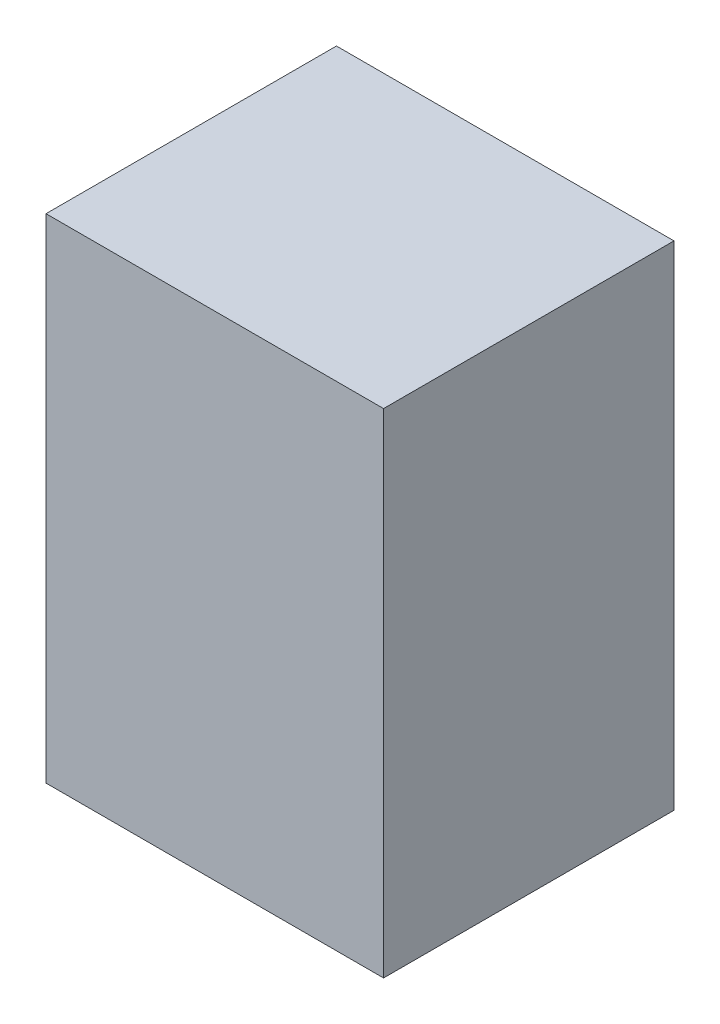
from build123d import *

# Parameters (mm, degrees)
SKETCH1_W           = 34.866263656
SKETCH1_H           = 50.939540762
BOSS_EXTRUDE1_DEPTH = 30


with BuildPart() as part:
    # Sketch1 → Boss-Extrude1 (new body)
    with BuildSketch(Plane.XY):
        Rectangle(SKETCH1_W, SKETCH1_H)
    extrude(amount=-BOSS_EXTRUDE1_DEPTH)


solid = part.part
